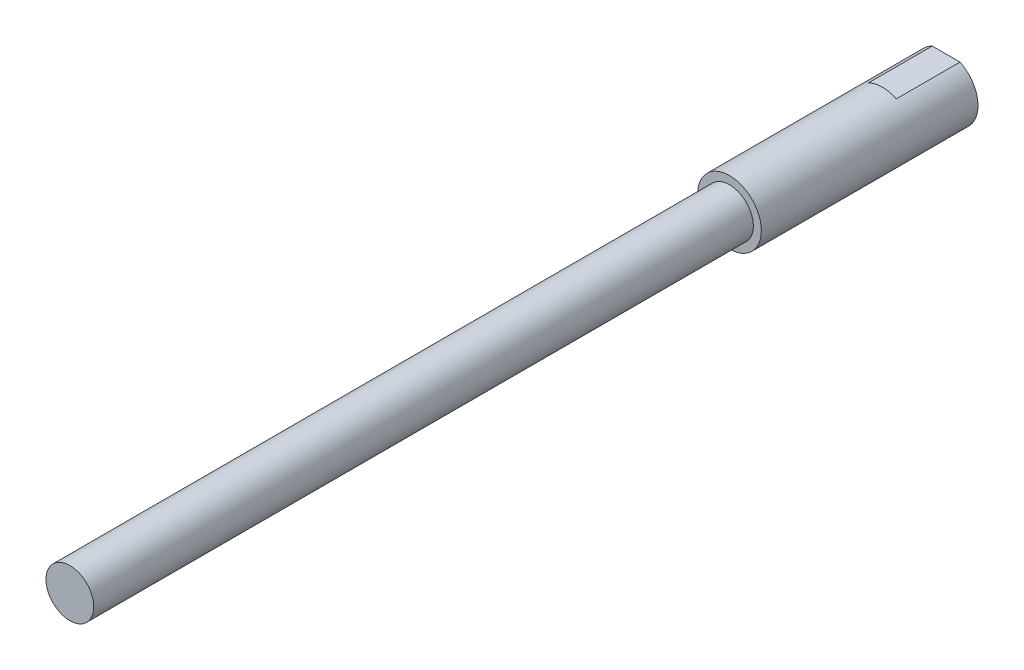
from build123d import *

# Parameters (mm, degrees)
SKETCH_1_R                   = 7.5
EXTRUDE_1_DEPTH              = 207
SKETCH_2_R                   = 10
EXTRUDE_2_DEPTH              = 68
SKETCH_3_OUTSIDE_W           = 77.29
SKETCH_3_OUTSIDE_H           = 77.29
SKETCH_3_OUTSIDE_W_2         = 23
SKETCH_3_OUTSIDE_H_2         = 18
CUT_EXTRUDE_1_DEPTH          = 20
HOLE_WIZARD_M8_1_D           = 6.8
HOLE_WIZARD_M8_1_DEPTH       = 18.25
HOLE_WIZARD_M8_1_CSINK_D     = 8.05
HOLE_WIZARD_M8_1_CSINK_ANGLE = 90
HOLE_WIZARD_M8_1_TIP         = 2.042926105


with BuildPart() as part:
    # 草图1 → 凸台-拉伸1 (new body)
    with BuildSketch(Plane.XY):
        Circle(SKETCH_1_R)
    extrude(amount=EXTRUDE_1_DEPTH)

    # 草图2 → 凸台-拉伸2 (add)
    with BuildSketch(Plane(origin=(0, 0, 0), x_dir=(-1, 0, 0), z_dir=(0, 0, -1))):
        Circle(SKETCH_2_R)
    extrude(amount=EXTRUDE_2_DEPTH)

    # 草图3 outside → 切除-拉伸1 (cut)
    with BuildSketch(Plane(origin=(0, 0, -68), x_dir=(-1, 0, 0), z_dir=(0, 0, -1))):
        Rectangle(SKETCH_3_OUTSIDE_W, SKETCH_3_OUTSIDE_H)
        Rectangle(SKETCH_3_OUTSIDE_W_2, SKETCH_3_OUTSIDE_H_2, mode=Mode.SUBTRACT)
    extrude(amount=-CUT_EXTRUDE_1_DEPTH, mode=Mode.SUBTRACT)

    # M8 螺纹孔1
    with Locations(Plane(origin=(0, 0, -68), x_dir=(-1, 0, 0), z_dir=(0, 0, -1))):
        with Locations((0, 0)):
            CounterSinkHole(HOLE_WIZARD_M8_1_D / 2, HOLE_WIZARD_M8_1_CSINK_D / 2, depth=HOLE_WIZARD_M8_1_DEPTH, counter_sink_angle=HOLE_WIZARD_M8_1_CSINK_ANGLE)
            with Locations((0, 0, -(HOLE_WIZARD_M8_1_DEPTH + HOLE_WIZARD_M8_1_TIP / 2))):  # 118° drill point
                Cone(0, HOLE_WIZARD_M8_1_D / 2, HOLE_WIZARD_M8_1_TIP, mode=Mode.SUBTRACT)


solid = part.part
